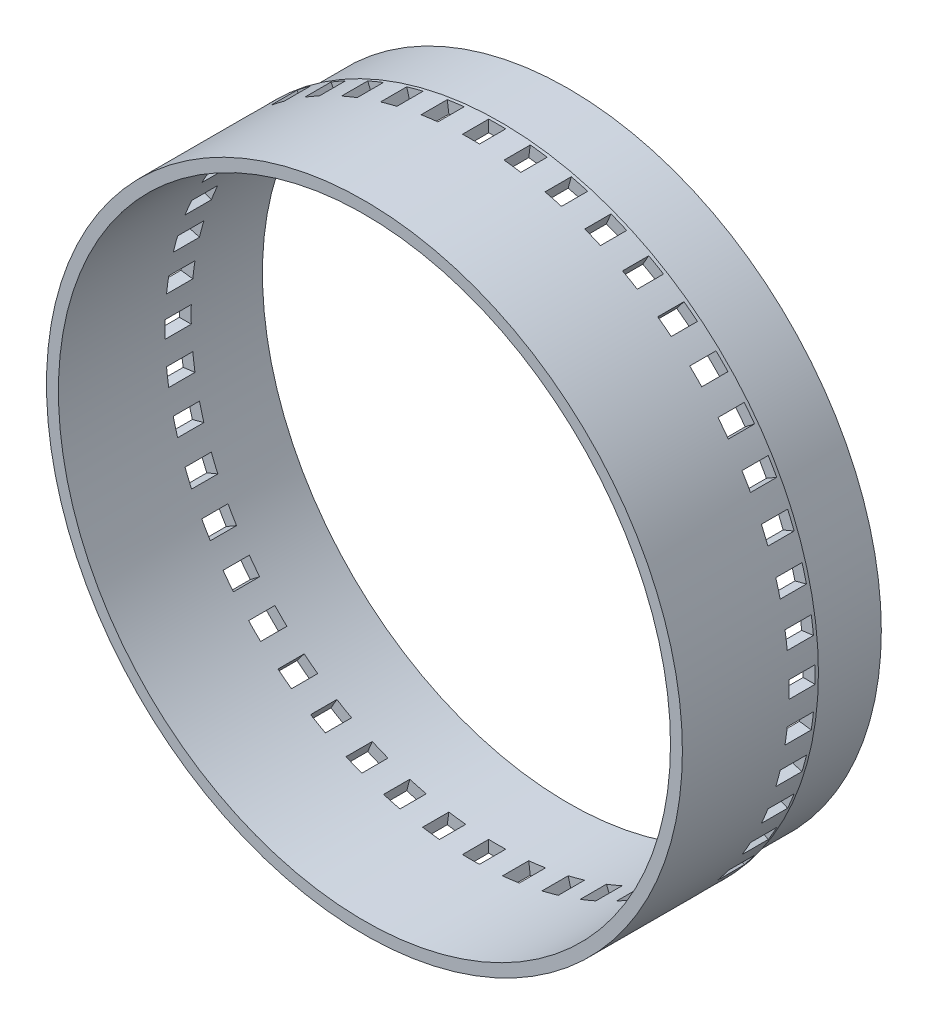
from build123d import *

# Parameters (mm, degrees)
SKETCH1_R           = 9.2
BOSS_EXTRUDE1_DEPTH = 2
SKETCH2_R           = 9.35
BOSS_EXTRUDE2_DEPTH = 4
SKETCH3_R           = 9
CUT_EXTRUDE1_DEPTH  = 13
SKETCH4_W           = 0.544798691
SKETCH4_H           = 0.771613806
CUT_EXTRUDE2_DEPTH  = 0.25
CIRPATTERN1_COUNT   = 48


with BuildPart() as part:
    # Sketch1 → Boss-Extrude1 (new body)
    with BuildSketch(Plane.XY):
        Circle(SKETCH1_R)
    extrude(amount=BOSS_EXTRUDE1_DEPTH)

    # Sketch2 → Boss-Extrude2 (add)
    with BuildSketch(Plane.XY.offset(2)):
        Circle(SKETCH2_R)
    extrude(amount=BOSS_EXTRUDE2_DEPTH)

    # Sketch3 → Cut-Extrude1 (cut)
    with BuildSketch(Plane.XY.offset(6)):
        Circle(SKETCH3_R)
    extrude(amount=-CUT_EXTRUDE1_DEPTH, mode=Mode.SUBTRACT)

    # Sketch4 → Cut-Extrude2 (cut, symmetric)
    with BuildSketch(Plane(origin=(0, 0, 0), x_dir=(1, 0, 0), z_dir=(0, 1, 0))):
        with Locations((-9.260365035, -2.481414608)):
            Rectangle(SKETCH4_W, SKETCH4_H)
    cut_extrude2 = extrude(amount=CUT_EXTRUDE2_DEPTH, both=True, mode=Mode.SUBTRACT)

    # CirPattern1: Cut-Extrude2 ×48 about axis
    cirpattern1_axis = Axis((0, 0, 0), (0, 0, 1))
    for i in range(1, CIRPATTERN1_COUNT):
        add(cut_extrude2.rotate(cirpattern1_axis, i * 360 / CIRPATTERN1_COUNT), mode=Mode.SUBTRACT)


solid = part.part
